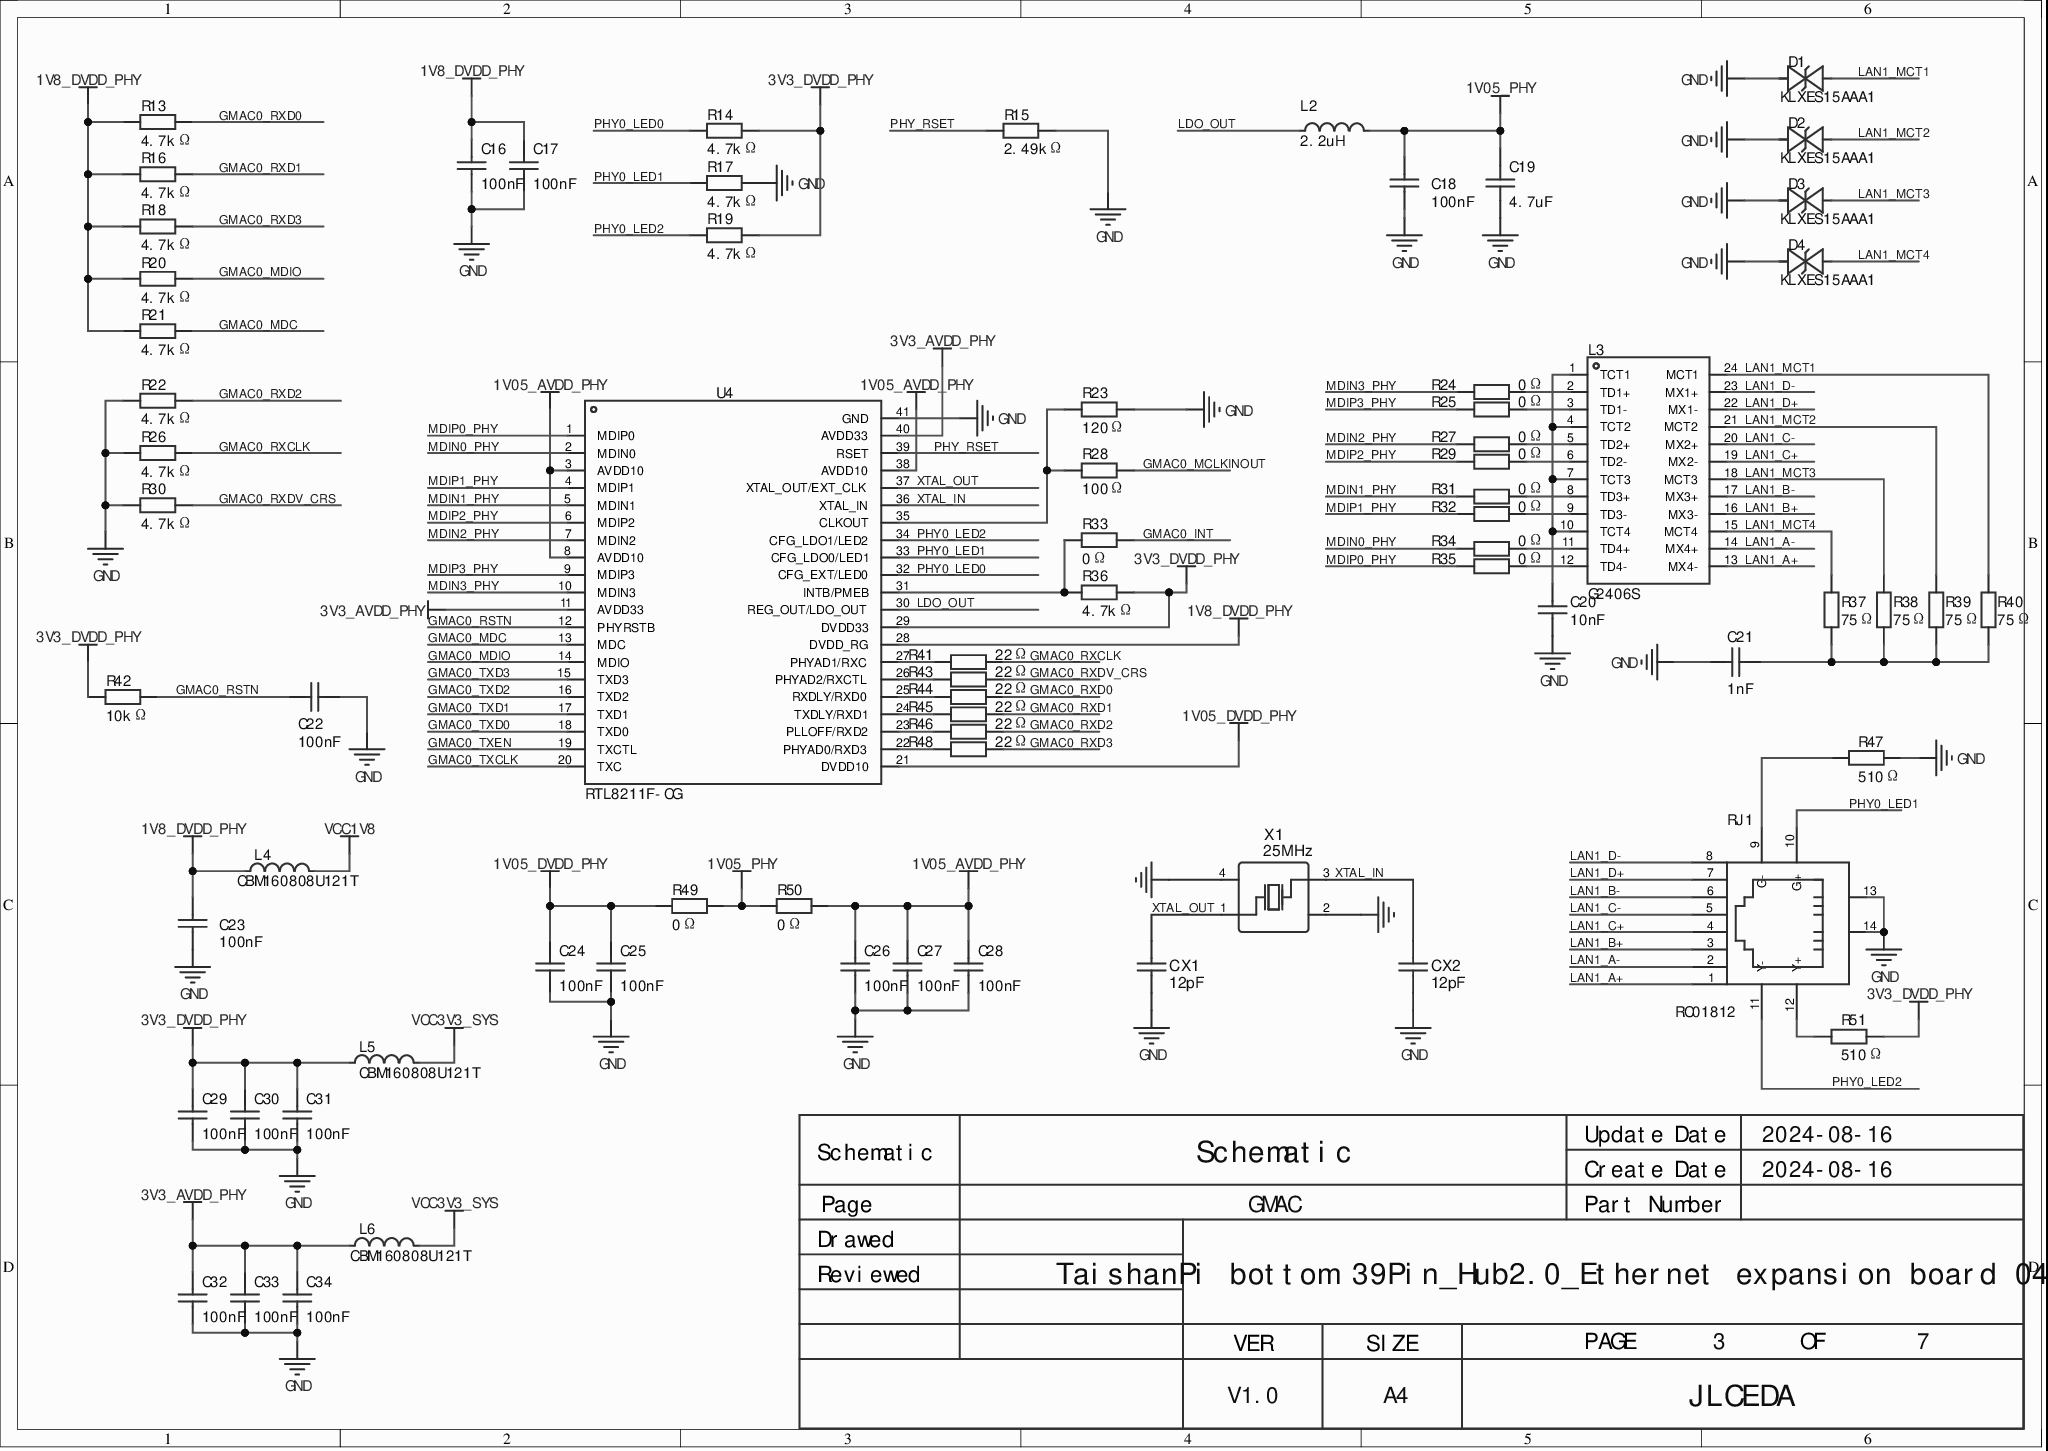
[diagram p0: MISC84334-4.SchDoc]
# Altium project MISC84334.PrjPcb (part 2 of 5)
## Sheet MISC84334-4.SchDoc (continued)
### Parts (continued)
C17  100nF  [R0402]
C18  100nF  [R0402]
C19  4.7uF  [R0402]
C20  10nF  [R1206]
C21  1nF  [R0402]
C22  100nF  [R0402]
C23  100nF  [R0402]
C24  100nF  [R0402]
C25  100nF  [R0402]
C26  100nF  [R0402]
C27  100nF  [R0402]
C28  100nF  [R0402]
C29  100nF  [R0402]
C30  100nF  [R0402]
C31  100nF  [R0402]
C32  100nF  [R0402]
C33  100nF  [R0402]
C34  100nF  [R0402]
CX1  12pF  [R0402]
CX2  12pF  [R0402]
D1  KLXES15AAA1  [D0402-BI]
D2  KLXES15AAA1  [D0402-BI]
D3  KLXES15AAA1  [D0402-BI]
D4  KLXES15AAA1  [D0402-BI]
L2  2.2uH  [IND-SMD_L2.5-W2.0_WPN252012H]
L3  G2406S  [SMD-24_L15.1-W7.1-P1.00-LS10.0-BL]
L4  CBM160808U121T  [L0603]
L5  CBM160808U121T  [L0603]
L6  CBM160808U121T  [L0603]
R13  4.7kΩ  [R0402]
R14  4.7kΩ  [R0402]
R15  2.49kΩ  [R0402]
R16  4.7kΩ  [R0402]
R17  4.7kΩ  [R0402]
R18  4.7kΩ  [R0402]
R19  4.7kΩ  [R0402]
R20  4.7kΩ  [R0402]
R21  4.7kΩ  [R0402]
R22  4.7kΩ  [R0402]
R23  120Ω  [R0402]
R24  0Ω  [R0402]
R25  0Ω  [R0402]
R26  4.7kΩ  [R0402]
R27  0Ω  [R0402]
R28  100Ω  [R0402]
R29  0Ω  [R0402]
R30  4.7kΩ  [R0402]
R31  0Ω  [R0402]
R32  0Ω  [R0402]
R33  0Ω  [R0402]
R34  0Ω  [R0402]
R35  0Ω  [R0402]
R36  4.7kΩ  [R0402]
R37  75Ω  [R0402]
R38  75Ω  [R0402]
R39  75Ω  [R0402]
R40  75Ω  [R0402]
R41  22Ω  [R0402]
R42  10kΩ  [R0402]
R43  22Ω  [R0402]
R44  22Ω  [R0402]
R45  22Ω  [R0402]
R46  22Ω  [R0402]
R47  510Ω  [R0402]
R48  22Ω  [R0402]
R49  0Ω  [R0402]
R50  0Ω  [R0402]
R51  510Ω  [R0402]
RJ1  RC01812  [RJ45-TH_RC01812]
U4  RTL8211F-CG  [WQFN-40_L5.0-W5.0-P0.4-BL-EP]
X1  25MHz  [OSC-SMD_4P-L3.2-W2.5-BL]

### Nets
1V05_AVDD_PHY: C26.2 C27.2 C28.2 R50.2 U4.3(AVDD10) U4.8(AVDD10) U4.38(AVDD10)
1V05_DVDD_PHY: C24.2 C25.2 R49.1 U4.21(DVDD10)
1V05_PHY: C18.2 C19.2 L2.2 R49.2 R50.1
1V8_DVDD_PHY: C16.2 C17.2 C23.2 L4.1 R13.1 R16.1 R18.1 R20.1 R21.1 U4.28(DVDD_RG)
3V3_AVDD_PHY: C32.2 C33.2 C34.2 L6.1 U4.11(AVDD33) U4.40(AVDD33)
3V3_DVDD_PHY: C29.2 C30.2 C31.2 L5.1 R14.2 R19.2 R36.2 R42.2 R51.1 U4.29(DVDD33)
GND: C16.1 C17.1 C18.1 C19.1 C20.1 C21.1 C22.1 C23.1 C24.1 C25.1 C26.1 C27.1 C28.1 C29.1 C30.1 C31.1 C32.1 C33.1 C34.1 CX1.1 CX2.1 D1.2(A) D2.2(A) D3.2(A) D4.2(A) R15.2 R17.2 R22.1 R23.2 R26.1 R30.1 R47.1 RJ1.13(SHELL) RJ1.14(SHELL) U4.41(GND) X1.2(GND) X1.4(GND)
VCC1V8: L4.2
VCC3V3_SYS: L5.2 L6.2
GMAC0_INT: R33.2
GMAC0_MCLKINOUT: R28.2
GMAC0_MDC: R21.2 U4.13(MDC)
GMAC0_MDIO: R20.2 U4.14(MDIO)
GMAC0_RSTN: C22.2 R42.1 U4.12(PHYRSTB)
GMAC0_RXCLK: R26.2 R41.2
GMAC0_RXD0: R13.2 R44.2
GMAC0_RXD1: R16.2 R45.2
GMAC0_RXD2: R22.2 R46.2
GMAC0_RXD3: R18.2 R48.2
GMAC0_RXDV_CRS: R30.2 R43.2
GMAC0_TXCLK: U4.20(TXC)
GMAC0_TXD0: U4.18(TXD0)
GMAC0_TXD1: U4.17(TXD1)
GMAC0_TXD2: U4.16(TXD2)
GMAC0_TXD3: U4.15(TXD3)
GMAC0_TXEN: U4.19(TXCTL)
LAN1_A+: L3.13(MX4-) RJ1.1
LAN1_A-: L3.14(MX4+) RJ1.2
LAN1_B+: L3.16(MX3-) RJ1.3
LAN1_B-: L3.17(MX3+) RJ1.6
LAN1_C+: L3.19(MX2-) RJ1.4
LAN1_C-: L3.20(MX2+) RJ1.5
LAN1_D+: L3.22(MX1-) RJ1.7
LAN1_D-: L3.23(MX1+) RJ1.8
LAN1_MCT1: D1.1(K) L3.24(MCT1) R40.2
LAN1_MCT2: D2.1(K) L3.21(MCT2) R39.2
LAN1_MCT3: D3.1(K) L3.18(MCT3) R38.2
LAN1_MCT4: D4.1(K) L3.15(MCT4) R37.2
LDO_OUT: L2.1 U4.30(REG_OUT/LDO_OUT)
MDIN0_PHY: R34.1 U4.2(MDIN0)
MDIN1_PHY: R31.1 U4.5(MDIN1)
MDIN2_PHY: R27.1 U4.7(MDIN2)
MDIN3_PHY: R24.1 U4.10(MDIN3)
MDIP0_PHY: R35.1 U4.1(MDIP0)
MDIP1_PHY: R32.1 U4.4(MDIP1)
MDIP2_PHY: R29.1 U4.6(MDIP2)
MDIP3_PHY: R25.1 U4.9(MDIP3)
PHY0_LED0: R14.1 U4.32(CFG_EXT/LED0)
PHY0_LED1: R17.1 RJ1.10(G+) U4.33(CFG_LDO0/LED1)
PHY0_LED2: R19.1 RJ1.11(Y-) U4.34(CFG_LDO1/LED2)
PHY_RSET: R15.1 U4.39(RSET)
XTAL_IN: CX2.2 U4.36(XTAL_IN) X1.3(OSC2)
XTAL_OUT: CX1.2 U4.37(XTAL_OUT/EXT_CLK) X1.1(OSC1)
NetC20_2: C20.2 L3.1(TCT1) L3.4(TCT2) L3.7(TCT3) L3.10(TCT4)
NetC21_2: C21.2 R37.1 R38.1 R39.1 R40.1
NetL3_2: L3.2(TD1+) R24.2
NetL3_3: L3.3(TD1-) R25.2
NetL3_5: L3.5(TD2+) R27.2
NetL3_6: L3.6(TD2-) R29.2
NetL3_8: L3.8(TD3+) R31.2
NetL3_9: L3.9(TD3-) R32.2
NetL3_11: L3.11(TD4+) R34.2
NetL3_12: L3.12(TD4-) R35.2
NetR23_1: R23.1 R28.1 U4.35(CLKOUT)
NetR33_1: R33.1 R36.1 U4.31(INTB/PMEB)
NetR41_1: R41.1 U4.27(PHYAD1/RXC)
NetR43_1: R43.1 U4.26(PHYAD2/RXCTL)
NetR44_1: R44.1 U4.25(RXDLY/RXD0)
NetR45_1: R45.1 U4.24(TXDLY/RXD1)
NetR46_1: R46.1 U4.23(PLLOFF/RXD2)
NetR47_2: R47.2 RJ1.9(G-)
NetR48_1: R48.1 U4.22(PHYAD0/RXD3)
NetR51_2: R51.2 RJ1.12(Y+)

### Notes on the sheet
- Update Date
- 2024-08-16
- Schematic
- Page
- GMAC
- Create Date
- Part Number
- Reviewed
- Drawed
- COMPANY_A TaishanPi bottom 39Pin_Hub2.0_Ethernet expansion board 0419 revision
- VER
- V1.0
- SIZE
- A4
- PAGE
- 3
- JLCEDA
- OF
- 7

### Library data of the parts
C16-C18 C22-C34 = CL05B104KO5NNNC: as C35 on sheet MISC84334-3; Device: CL05B104KO5NNNC; Symbol: CL05B104KO5NNNC; LCSC Part Name: 100nF ±10% 16V; SupplierPart: C1525; ManufacturerPart: CL05B104KO5NNNC; Supplier Footprint: 0402; JLCPCB Part Class: Basic library; Datasheet: https://atta.szlcsc.com/upload/public/pdf/source/20160103/1457707674891.pdf; Supplier: LCSC; ConvertToPcb: yes; FootprintName: R0402; Value: 100nF
C19 = CL05A475MQ5NRNC: Capacitance:4.7uF;Tolerance:±20%;Rated voltage:6.3V;Dielectric(Temp. coefficient):X5R;; Manufacturer: SAMSUNG(三星); Symbol: CL05A475MQ5NRNC_C307423; AddInBom: yes; ModelId: 36a51122f27c49738f86b3bfa98863e0; ModelName: C0402_L1.0-W0.5-H0.5; ModelTransform: 39.37,19.685,0,0,0,0,0,0,0; Tolerance: ±20%; Voltage Rated: 6.3V; Temperature Coefficient: X5R; Device: CL05A475MQ5NRNC; LCSC Part Name: 4.7uF ±20% 6.3V; SupplierPart: C307423; ManufacturerPart: CL05A475MQ5NRNC; Supplier Footprint: 0402; JLCPCB Part Class: Extended library; Datasheet: https://atta.szlcsc.com/upload/public/pdf/source/20181010/C307423_0E0C4E35F3A09F81C2E5C84E00499E42.pdf; Supplier: LCSC; ConvertToPcb: yes; FootprintName: R0402; Value: 4.7uF
C20 = CC0402KRX7R9BB103: Capacitance:10nF;Tolerance:±10%;Rated voltage:50V;Dielectric(Temp. coefficient):X7R;; Manufacturer: HUI JU(汇聚); AddInBom: yes; ModelId: 36a51122f27c49738f86b3bfa98863e0; ModelName: C0402_L1.0-W0.5-H0.5; ModelTransform: 39.37,19.685,0,0,0,0,0,0,0; Tolerance: ±10%; Voltage Rated: 50V; Temperature Coefficient: X7R; Supplier Part: C976252; Device: CC0402KRX7R9BB103; Symbol: CC0402KRX7R9BB103; LCSC Part Name: 10nF ±10% 50V; ManufacturerPart: CC0402KRX7R9BB103; Supplier Footprint: 0402; JLCPCB Part Class: Extended library; Datasheet: https://atta.szlcsc.com/upload/public/pdf/source/20151201/1457707601869.pdf; Supplier: LCSC; ConvertToPcb: yes; FootprintName: R1206; Value: 10nF
C21 = CC0402KRX7R9BB102: Capacitance:1nF;Tolerance:±10%;Rated voltage:50V;Dielectric(Temp. coefficient):X7R;; Manufacturer: YAGEO(国巨); AddInBom: yes; ModelId: 36a51122f27c49738f86b3bfa98863e0; ModelName: C0402_L1.0-W0.5-H0.5; ModelTransform: 39.37,19.685,0,0,0,0,0,0,0; Tolerance: ±10%; Voltage Rated: 50V; Temperature Coefficient: X7R; Symbol: CC0402KRX7R9BB102; Device: CC0402KRX7R9BB102; Supplier: LCSC; Manufacturer Part: CC0402KRX7R9BB102; Value: 1nF; Supplier Part: C106205; JLCPCB Part Class: Extended library; LCSC Part Name: 1nF ±10% 50V; Supplier Footprint: 0402; Datasheet: https://atta.szlcsc.com/upload/public/pdf/source/20171226/C106205_15142609593391205665.pdf; ConvertToPcb: yes; FootprintName: R0402
CX1 CX2 = 0402CG120J500NT: Capacitance:12pF;Tolerance:±5%;Rated voltage:50V;Dielectric(Temp. coefficient):C0G;; Manufacturer: FH(风华); Origin Footprint: C0402; Symbol: 18pF; Convert to PCB: yes; ModelId: 36a51122f27c49738f86b3bfa98863e0; ModelName: C0402_L1.0-W0.5-H0.5; ModelTransform: 39.37,19.685,0,0,0,0,0,0,0; Tolerance: ±5%; Voltage Rated: 50V; Temperature Coefficient: C0G; JLCPCB Part Class: Basic Part; Device: 0402CG120J500NT; Add into BOM: yes; LCSC Part Name: 12pF ±5% 50V; SupplierPart: C1547; ManufacturerPart: 0402CG120J500NT; Supplier Footprint: 0402; Datasheet: https://atta.szlcsc.com/upload/public/pdf/source/20200305/C486355_26A10D38EF8C2A5C37091D0039909270.pdf; Supplier: LCSC; FootprintName: R0402; Value: 12pF
D1-D4 = KLXES15AAA1: Polarity:Bidirectional;Reverse standoff voltage(Vrwm):5V;Clamping voltage(Vc)@Ipp:40V;; Manufacturer: KUU; AddInBom: yes; ModelId: 62a80a189f1b46df8ba79817b730b378; ModelName: D0402_L1.0-W0.5-H0.5; ModelTransform: 39.37,19.685,0,0,0,0,0,0,0; Reverse Stand-Off Voltage (Vrwm): 5V; Clamping Voltage@Ipp: 40V; Device: KLXES15AAA1; Symbol: KLXES15AAA1; LCSC Part Name: KLXES15AAA1; SupplierPart: C2892490; ManufacturerPart: KLXES15AAA1; Supplier Footprint: 0402; JLCPCB Part Class: Extended Part; Datasheet: https://atta.szlcsc.com/upload/public/pdf/source/20210908/40FD94D5521B4EF0ED53BC030E77ED53.pdf; Supplier: LCSC; ConvertToPcb: yes; FootprintName: D0402-BI; Polarity: Bidirectional
L2 = WPN252012H2R2MT: Type:-;Inductance:2.2uH;Tolerance:±20%;Rated current:1.9A;Saturation current(Isat):3A;; Manufacturer: Sunlord(顺络); Symbol: SWPA3015S2R2MT; AddInBom: yes; ModelId: 7ae8e774cfcf498ea5119a488d0de531; ModelName: IND-SMD_L2.5-W2.0-H1.2-252012; ModelTransform: 78.74,99.2124,0,90,0,0,0,0,0; Tolerance: ±20%; Rated Current: 1.9A; Saturation Current (Isat): 3A; DC Resistance (DCR): 120mΩ; Device: WPN252012H2R2MT; LCSC Part Name: 2.2uH ±20% 3A; SupplierPart: C98350; ManufacturerPart: WPN252012H2R2MT; Supplier Footprint: SMD; JLCPCB Part Class: Extended Part; Datasheet: https://atta.szlcsc.com/upload/public/pdf/source/20210916/5D33DED32780FEB7D0AA8BED8FC93477.pdf; Supplier: LCSC; ConvertToPcb: yes; FootprintName: IND-SMD_L2.5-W2.0_WPN252012H; Type: -; Value: 2.2uH; Ratings: -
L3 = G2406S_C507595: Winding sets:4;; Manufacturer: CND-tek(磁联达); AddInBom: yes; ModelId: fb36f8447ed64154860c45d69daaf8fa; ModelName: SMD-24_L15.1-W7.1-H4.5-P1.00-LS10.0-BL; ModelTransform: 594.487,393.7,0,0,0,0,0,0,0; Number of Loop: 4; Turns Ratio: 1:1; Device: G2406S_C507595; Symbol: G2406S_C507595; LCSC Part Name: 单口千兆网络隔离变压器; SupplierPart: C507595; ManufacturerPart: G2406S; Supplier Footprint: SMD-24P; JLCPCB Part Class: Extended library; Datasheet: https://atta.szlcsc.com/upload/public/pdf/source/20230307/FCB9470D48A21F045F41A5A00FC9CB7C.pdf; Supplier: LCSC; ConvertToPcb: yes; FootprintName: SMD-24_L15.1-W7.1-P1.00-LS10.0-BL
L4-L6 = CBM160808U121T: Impedance@test frequency:120Ω@100MHz;Tolerance:±25%;DC resistance(RDC):65mΩ;; Manufacturer: FH(风华); AddInBom: yes; ModelId: 2bc5ec593d464d6ba9807aec0b5673c2; ModelName: L0603_L1.6-W0.8-H0.5_BEAD; ModelTransform: 62.992,31.496,0,180,0,0,0.094,0.629,0; Tolerance: ±25%; DC Resistance: 65mΩ; Current Rating: 2A; Circuits: 1; Device: CBM160808U121T; Symbol: CBM160808U121T; LCSC Part Name: 单路 0603磁珠 阻抗120Ω@100MHz; SupplierPart: C62708; ManufacturerPart: CBM160808U121T; Supplier Footprint: 0603; JLCPCB Part Class: Extended library; Datasheet: https://atta.szlcsc.com/upload/public/pdf/source/20151203/1457707610455.pdf; Supplier: LCSC; ConvertToPcb: yes; FootprintName: L0603; Impedance @ Frequency: 120Ω@100MHz
R13 R14 R16-R22 R26 R30 R36 = 0402WGF4701TCE: as R52 on sheet MISC84334-3; Symbol: 0402WGF4701TCE; Device: 0402WGF4701TCE; Supplier: LCSC; Manufacturer Part: 0402WGF4701TCE; Supplier Part: C25900; Value: 4.7kΩ; JLCPCB Part Class: Basic library; LCSC Part Name: 4.7kΩ ±1% 62.5mW; Supplier Footprint: 0402; Datasheet: https://atta.szlcsc.com/upload/public/pdf/source/20200306/C422600_1E6D84923E4A46A82E41ADD87F860B5C.pdf; ConvertToPcb: yes; FootprintName: R0402; Type: Thick film resistor; Operating Temperature Range: -55℃~+155℃
R15 = RC0402FR-072K49L: Resistor type:Thick film resistor;Resistance:2.49kΩ;Tolerance:±1%;Power:62.5mW;; Manufacturer: YAGEO(国巨); AddInBom: yes; ModelId: 671aefced39d4c318694bba8bd8efd39; ModelName: R0402_L1.0-W0.5-H0.5; ModelTransform: 39.37,19.685,0,0,0,0,0,0.0005,0; Tolerance: ±1%; Power(Watts): 62.5mW; Temperature Coefficient: ±100ppm/℃; Overload Voltage (Max): 50V; Device: RC0402FR-072K49L; Symbol: RC0402FR-072K49L; LCSC Part Name: 厚膜电阻 2.49kΩ ±1% 62.5mW; SupplierPart: C145071; ManufacturerPart: RC0402FR-072K49L; Supplier Footprint: 0402; JLCPCB Part Class: Extended library; Datasheet: https://atta.szlcsc.com/upload/public/pdf/source/20171221/C145071_15138311814201195405.pdf; Supplier: LCSC; ConvertToPcb: yes; FootprintName: R0402; Type: Thick film resistor; Value: 2.49kΩ; Operating Temperature Range: -55℃~+155℃
R23 = RC0402FR-07120RL: Resistor type:Thick film resistor;Resistance:120Ω;Tolerance:±1%;Power:62.5mW;; Manufacturer: YAGEO(国巨); AddInBom: yes; ModelId: 671aefced39d4c318694bba8bd8efd39; ModelName: R0402_L1.0-W0.5-H0.5; ModelTransform: 39.37,19.685,0,0,0,0,0,0.0005,0; Tolerance: ±1%; Power(Watts): 62.5mW; Temperature Coefficient: ±100ppm/℃; Overload Voltage (Max): 50V; Device: RC0402FR-07120RL; Symbol: RC0402FR-07120RL; LCSC Part Name: 120Ω ±1% 62.5mW; SupplierPart: C114758; ManufacturerPart: RC0402FR-07120RL; Supplier Footprint: 0402; JLCPCB Part Class: Extended library; Datasheet: https://atta.szlcsc.com/upload/public/pdf/source/20170912/C114758_1505207815629963476.pdf; Supplier: LCSC; ConvertToPcb: yes; FootprintName: R0402; Type: Thick film resistor; Value: 120Ω; Operating Temperature Range: -55℃~+155℃
R24 R25 R27 R29 R31 R32 R34 R35 = 0402WGJ0000TCE: Resistor type:Thick film resistor;Resistance:0Ω;Tolerance:±5%;Power:62.5mW;; Manufacturer: UNI-ROYAL(厚声); AddInBom: yes; ModelId: 671aefced39d4c318694bba8bd8efd39; ModelName: R0402_L1.0-W0.5-H0.5; ModelTransform: 39.37,19.685,0,0,0,0,0,0.0005,0; Tolerance: ±5%; Power(Watts): 62.5mW; Overload Voltage (Max): 50V; Device: 0402WGJ0000TCE; Symbol: 0402WGJ0000TCE; LCSC Part Name: 0Ω ±5% 62.5mW; SupplierPart: C21376; ManufacturerPart: 0402WGJ0000TCE; Supplier Footprint: 0402; JLCPCB Part Class: Extended library; Datasheet: https://atta.szlcsc.com/upload/public/pdf/source/20200306/C422600_1E6D84923E4A46A82E41ADD87F860B5C.pdf; Supplier: LCSC; ConvertToPcb: yes; FootprintName: R0402; Type: Thick film resistor; Value: 0Ω; Operating Temperature Range: -55℃~+155℃
R28 = 0402WGF1000TCE: Resistor type:Thick film resistor;Resistance:100Ω;Tolerance:±1%;Power:62.5mW;; Manufacturer: UNI-ROYAL(厚声); AddInBom: yes; ModelId: 671aefced39d4c318694bba8bd8efd39; ModelName: R0402_L1.0-W0.5-H0.5; ModelTransform: 39.37,19.685,0,0,0,0,0,0.0005,0; Tolerance: ±1%; Power(Watts): 62.5mW; Temperature Coefficient: ±200ppm/℃; Overload Voltage (Max): 50V; Device: 0402WGF1000TCE; Symbol: 0402WGF1000TCE; LCSC Part Name: 100Ω ±1% 62.5mW; SupplierPart: C25076; ManufacturerPart: 0402WGF1000TCE; Supplier Footprint: 0402; JLCPCB Part Class: Basic library; Datasheet: https://atta.szlcsc.com/upload/public/pdf/source/20200306/C422600_1E6D84923E4A46A82E41ADD87F860B5C.pdf; Supplier: LCSC; ConvertToPcb: yes; FootprintName: R0402; Type: Thick film resistor; Value: 100Ω; Operating Temperature Range: -55℃~+155℃
R33 R49 R50 = 0402WGF0000TCE: Resistor type:Thick film resistor;Resistance:0Ω;Tolerance:±1%;Power:62.5mW;; Manufacturer: UNI-ROYAL(厚声); AddInBom: yes; ModelId: 671aefced39d4c318694bba8bd8efd39; ModelName: R0402_L1.0-W0.5-H0.5; ModelTransform: 39.37,19.685,0,0,0,0,0,0.0005,0; Tolerance: ±1%; Power(Watts): 62.5mW; Temperature Coefficient: ±800ppm/℃; Overload Voltage (Max): 50V; Symbol: 0402WGF0000TCE; Device: 0402WGF0000TCE; Supplier: LCSC; Manufacturer Part: 0402WGF0000TCE; Supplier Part: C17168; Value: 0Ω; JLCPCB Part Class: Basic library; LCSC Part Name: 0Ω ±1% 62.5mW; Supplier Footprint: 0402; Datasheet: https://atta.szlcsc.com/upload/public/pdf/source/20200306/C422600_1E6D84923E4A46A82E41ADD87F860B5C.pdf; ConvertToPcb: yes; FootprintName: R0402; Type: Thick film resistor; Operating Temperature Range: -55℃~+155℃
R37-R40 = 0402WGF750JTCE: Resistor type:Thick film resistor;Resistance:75Ω;Tolerance:±1%;Power:62.5mW;; Manufacturer: UNI-ROYAL(厚声); AddInBom: yes; ModelId: 671aefced39d4c318694bba8bd8efd39; ModelName: R0402_L1.0-W0.5-H0.5; ModelTransform: 39.37,19.685,0,0,0,0,0,0.0005,0; Tolerance: ±1%; Power(Watts): 62.5mW; Temperature Coefficient: ±100ppm/℃; Overload Voltage (Max): 50V; Device: 0402WGF750JTCE; Symbol: 0402WGF750JTCE; LCSC Part Name: 75Ω ±1% 62.5mW; SupplierPart: C25133; ManufacturerPart: 0402WGF750JTCE; Supplier Footprint: 0402; JLCPCB Part Class: Basic library; Datasheet: https://atta.szlcsc.com/upload/public/pdf/source/20200306/C422600_1E6D84923E4A46A82E41ADD87F860B5C.pdf; Supplier: LCSC; ConvertToPcb: yes; FootprintName: R0402; Type: Thick film resistor; Value: 75Ω; Operating Temperature Range: -55℃~+155℃
R41 R43-R46 R48 = 0402WGF220JTCE: Resistor type:Thick film resistor;Resistance:22Ω;Tolerance:±1%;Power:62.5mW;; Manufacturer: UNI-ROYAL(厚声); AddInBom: yes; ModelId: 671aefced39d4c318694bba8bd8efd39; ModelName: R0402_L1.0-W0.5-H0.5; ModelTransform: 39.37,19.685,0,0,0,0,0,0.0005,0; Tolerance: ±1%; Power(Watts): 62.5mW; Temperature Coefficient: ±200ppm/℃; Overload Voltage (Max): 50V; Device: 0402WGF220JTCE; Symbol: 0402WGF220JTCE; LCSC Part Name: 22Ω ±1% 62.5mW; SupplierPart: C25092; ManufacturerPart: 0402WGF220JTCE; Supplier Footprint: 0402; JLCPCB Part Class: Basic library; Datasheet: https://atta.szlcsc.com/upload/public/pdf/source/20200306/C422600_1E6D84923E4A46A82E41ADD87F860B5C.pdf; Supplier: LCSC; ConvertToPcb: yes; FootprintName: R0402; Type: Thick film resistor; Value: 22Ω; Operating Temperature Range: -55℃~+155℃
R42 = 0402WGF1002TCE: Resistor type:Thick film resistor;Resistance:10kΩ;Tolerance:±1%;Power:62.5mW;; Manufacturer: UNI-ROYAL(厚声); AddInBom: yes; ModelId: 671aefced39d4c318694bba8bd8efd39; ModelName: R0402_L1.0-W0.5-H0.5; ModelTransform: 39.37,19.685,0,0,0,0,0,0.0005,0; Tolerance: ±1%; Power(Watts): 62.5mW; Temperature Coefficient: ±100ppm/℃; Overload Voltage (Max): 50V; Symbol: 0402WGF1002TCE; Device: 0402WGF1002TCE; Supplier: LCSC; Manufacturer Part: 0402WGF1002TCE; Supplier Part: C25744; Value: 10kΩ; JLCPCB Part Class: Basic library; LCSC Part Name: 10kΩ ±1% 62.5mW; Supplier Footprint: 0402; Datasheet: https://atta.szlcsc.com/upload/public/pdf/source/20200306/C422600_1E6D84923E4A46A82E41ADD87F860B5C.pdf; ConvertToPcb: yes; FootprintName: R0402; Type: Thick film resistor; Operating Temperature Range: -55℃~+155℃
R47 R51 = RC0402JR-07510RL: Resistor type:Thick film resistor;Resistance:510Ω;Tolerance:±5%;Power:62.5mW;; Manufacturer: YAGEO(国巨); AddInBom: yes; ModelId: 671aefced39d4c318694bba8bd8efd39; ModelName: R0402_L1.0-W0.5-H0.5; ModelTransform: 39.37,19.685,0,0,0,0,0,0.0005,0; Tolerance: ±5%; Power(Watts): 62.5mW; Temperature Coefficient: ±100ppm/℃; Overload Voltage (Max): 50V; Device: RC0402JR-07510RL; Symbol: RC0402JR-07510RL; LCSC Part Name: 510Ω ±5% 62.5mW; SupplierPart: C137860; ManufacturerPart: RC0402JR-07510RL; Supplier Footprint: 0402; JLCPCB Part Class: Extended library; Datasheet: https://atta.szlcsc.com/upload/public/pdf/source/20171107/C137860_15100515269831096793.pdf; Supplier: LCSC; ConvertToPcb: yes; FootprintName: R0402; Type: Thick film resistor; Value: 510Ω; Operating Temperature Range: -55℃~+155℃
RJ1 = RC01812: RCH-SP32-TP(with LED, no spring)1U LED length 2.6; Manufacturer: RCH(瑞川); AddInBom: yes; ModelId: 3f949edb5ed54b24a87015b7caf84239; ModelTransform: 637.796,669.291,0,0,0,0,0,139.764,-165.354; Device: RC01812; LCSC Part Name: RC01812; SupplierPart: C708645; ManufacturerPart: RC01812; Supplier Footprint: -; JLCPCB Part Class: Extended library; Datasheet: https://atta.szlcsc.com/upload/public/pdf/source/20200728/C708645_B766D64FA5E244BAC68F6632C426138D.pdf; Supplier: LCSC; ConvertToPcb: yes; SymbolName: RC01812; FootprintName: RJ45-TH_RC01812; ModelName: RJ45-TH_RC01812
U4 = RTL8211F-CG: Application:-;Channels:-;Interface type:-;; Manufacturer: REALTEK(瑞昱); AddInBom: yes; ModelId: 0596a0bbfbbe4c109fc43a604c259f16; ModelTransform: 197.6374,197.6374,0,0,0,0,0,0,0; Device: RTL8211F-CG; Symbol: RTL8211F-CG; LCSC Part Name: RTL8211F-CG; SupplierPart: C187932; ManufacturerPart: RTL8211F-CG; Supplier Footprint: WQFN-40-EP(5x5); JLCPCB Part Class: Extended library; Datasheet: https://atta.szlcsc.com/upload/public/pdf/source/20190902/C187932_1913F3711F05FE1324DF2946D70D648D.pdf; Supplier: LCSC; ConvertToPcb: yes; FootprintName: WQFN-40_L5.0-W5.0-P0.4-BL-EP; ModelName: WQFN-40_L5.0-W5.0-P0.4-BL-EP; Application Function: -; Number of Channels: -; Interface: -
X1 = X322525MOB4SI: Frequency:25MHz;Frequency tolerance:±10ppm;Load capacitance:12pF;; Manufacturer: YXC(扬兴晶振); Origin Footprint: CRYSTAL-SMD_4P-L2.5-W2.0-BL; Convert to PCB: yes; ModelId: ae22b8d143894765bc8100c37cb6356f; ModelName: OSC-SMD_4P-L3.2-W2.5-H1.0; ModelTransform: 125.984,98.425,0,0,0,0,0,0,0; Crystal Type: SMD passive crystal; Frequency Tolerance: ±10ppm; Frequency Stability: ±30ppm; Load Capacitance: 12pF; JLCPCB Part Class: Basic Part; Device: X322525MOB4SI; Symbol: 25MHz; Add into BOM: yes; LCSC Part Name: 25MHz ±10ppm 12pF YSX321SL; SupplierPart: C9006; ManufacturerPart: X322525MOB4SI; Supplier Footprint: SMD3225-4P; Datasheet: https://atta.szlcsc.com/upload/public/pdf/source/20210329/C112971_1F611BDC486E193C1706F6D8EB5AA189.pdf; Supplier: LCSC; FootprintName: OSC-SMD_4P-L3.2-W2.5-BL; Value: 25MHz; Operating Temperature: -40℃~+85℃